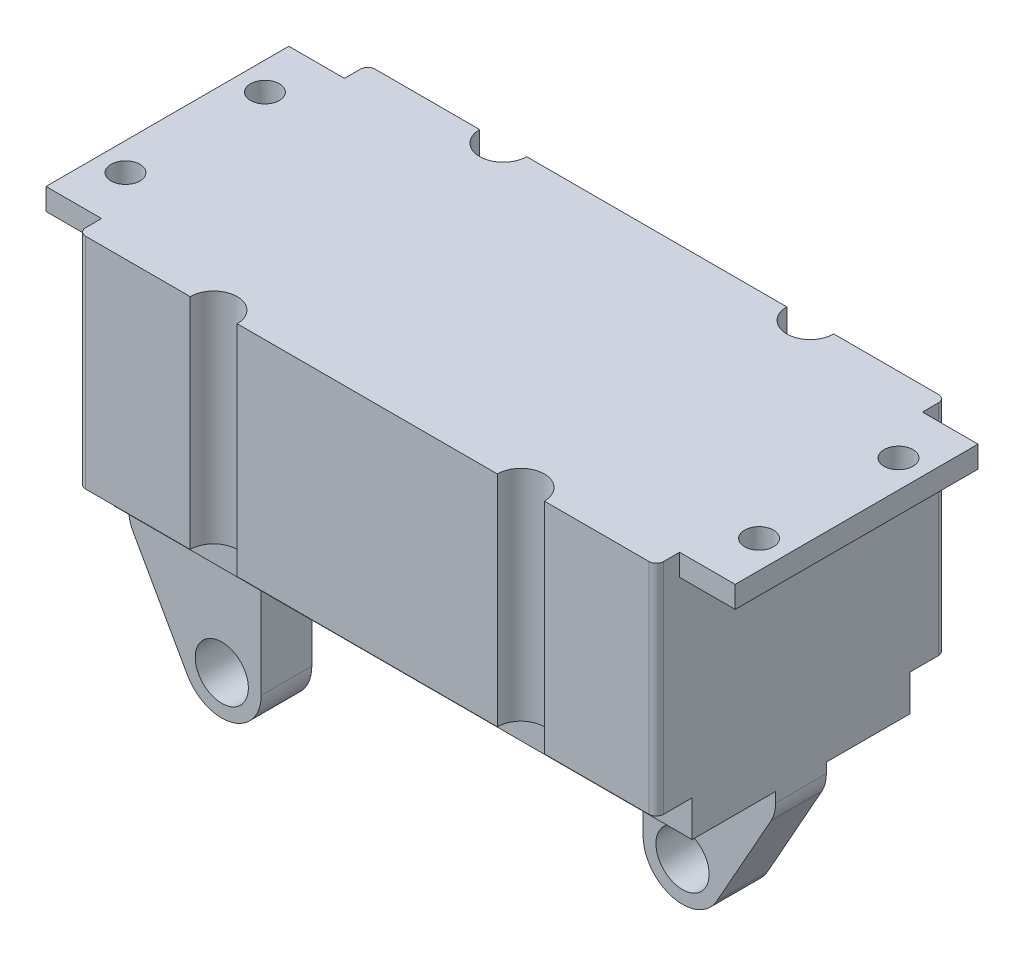
from build123d import *

# Parameters (mm, degrees)
SKETCH1_W           = 79.884759576
SKETCH1_H           = 30.264710677
BOSS_EXTRUDE1_DEPTH = 20
SKETCH2_W           = 79.884759576
SKETCH2_H           = 30.088424062
BOSS_EXTRUDE2_DEPTH = 5
SKETCH3_R           = 3.245829629
CUT_EXTRUDE1_DEPTH  = 47
FILLET1_R           = 1
SKETCH4_R           = 3.674588618
BOSS_EXTRUDE3_DEPTH = 7
SKETCH5_R           = 3.674588618
BOSS_EXTRUDE4_DEPTH = 3.5
SKETCH6_W           = 7.683150555
SKETCH6_H           = 33.560004606
SKETCH6_R           = 2
BOSS_EXTRUDE5_DEPTH = 3


with BuildPart() as part:
    # Sketch1 → Boss-Extrude1 (new, symmetric)
    with BuildSketch(Plane.XY):
        with Locations((0, 50.939731052)):
            Rectangle(SKETCH1_W, SKETCH1_H)
    extrude(amount=BOSS_EXTRUDE1_DEPTH, both=True)

    # Sketch2 → Boss-Extrude2 (add)
    with BuildSketch(Plane.XZ.offset(-35.807375713)):
        Rectangle(SKETCH2_W, SKETCH2_H)
    extrude(amount=BOSS_EXTRUDE2_DEPTH)

    # Sketch3 → Cut-Extrude1 (cut)
    with BuildSketch(Plane(origin=(0, 66.07208639, 0), x_dir=(1, 0, 0), z_dir=(0, 1, 0))):
        with Locations((-21.223926361, 20)):
            Circle(SKETCH3_R)
        with Locations((21.223926361, 20)):
            Circle(SKETCH3_R)
        with Locations((21.223926361, -20)):
            Circle(SKETCH3_R)
        with Locations((-21.223926361, -20)):
            Circle(SKETCH3_R)
    extrude(amount=-CUT_EXTRUDE1_DEPTH, mode=Mode.SUBTRACT)

    # Fillet1
    fillet1_edges = [part.edges().sort_by_distance(p)[0] for p in [
        (-39.942379788, 50.939731051, 20),
        (39.942379788, 50.939731051, 20),
        (-39.942379788, 50.939731051, -20),
        (39.942379788, 50.939731051, -20),
    ]]
    fillet(fillet1_edges, radius=FILLET1_R)

    # Sketch4 → Boss-Extrude3 (add)
    with BuildSketch(Plane.XY.offset(13.044212031)):
        with BuildLine():
            Line((-39.942379788, 30.807375713), (-39.942379788, 29.427732571))
            ThreePointArc((-39.942379788, 29.427732571), (-39.780068199, 28.164098588), (-39.303671451, 26.98250558))
            Line((-39.303671451, 26.98250558), (-31.815081757, 13.625903547))
            ThreePointArc((-31.815081757, 13.625903547), (-25.689559132, 11.020522164), (-21.620670757, 16.288746435))
            Line((-21.620670757, 16.288746435), (-21.620670757, 30.807375713))
            Line((-21.620670757, 30.807375713), (-39.942379788, 30.807375713))
        make_face()
        with Locations((-27.065651732, 16.288746435)):
            Circle(SKETCH4_R, mode=Mode.SUBTRACT)
    boss_extrude3 = extrude(amount=-BOSS_EXTRUDE3_DEPTH)

    # Mirror1: Boss-Extrude3 across plane
    add(boss_extrude3.mirror(Plane.XY))

    # Sketch5 → Boss-Extrude4 (add, symmetric)
    with BuildSketch(Plane.XY):
        with BuildLine():
            Line((21.620670757, 16.288746435), (21.620670757, 30.807375713))
            Line((21.620670757, 30.807375713), (39.942379788, 30.807375713))
            Line((39.942379788, 30.807375713), (39.942379788, 29.427732571))
            ThreePointArc((39.942379788, 29.427732571), (39.780068199, 28.164098588), (39.303671451, 26.98250558))
            Line((39.303671451, 26.98250558), (31.815081757, 13.625903547))
            ThreePointArc((31.815081757, 13.625903547), (25.689559132, 11.020522164), (21.620670757, 16.288746435))
        make_face()
        with Locations((27.065651732, 16.288746435)):
            Circle(SKETCH5_R, mode=Mode.SUBTRACT)
    extrude(amount=BOSS_EXTRUDE4_DEPTH, both=True)

    # Sketch6 → Boss-Extrude5 (add)
    # profile 1 of 2: a face of its own
    with BuildSketch(Plane(origin=(0, 66.07208639, 0), x_dir=(1, 0, 0), z_dir=(0, 1, 0))):
        with Locations((-43.783955066, 0)):
            Rectangle(SKETCH6_W, SKETCH6_H)
        with Locations(Location((-43.783955066, 9.635125017, 0), (0, 0, 270))):
            Circle(SKETCH6_R, mode=Mode.SUBTRACT)
        with Locations(Location((-43.783955066, -9.635125017, 0), (0, 0, 90))):
            Circle(SKETCH6_R, mode=Mode.SUBTRACT)
    # profile 2 of 2: a face of its own
    with BuildSketch(Plane(origin=(0, 66.07208639, 0), x_dir=(1, 0, 0), z_dir=(0, 1, 0))):
        with Locations((43.783955066, 0)):
            Rectangle(SKETCH6_W, SKETCH6_H)
        with Locations(Location((43.783955066, -9.635125017, 0), (0, 0, 270))):
            Circle(SKETCH6_R, mode=Mode.SUBTRACT)
        with Locations(Location((43.783955066, 9.635125017, 0), (0, 0, 90))):
            Circle(SKETCH6_R, mode=Mode.SUBTRACT)
    extrude(amount=-BOSS_EXTRUDE5_DEPTH)


solid = part.part
